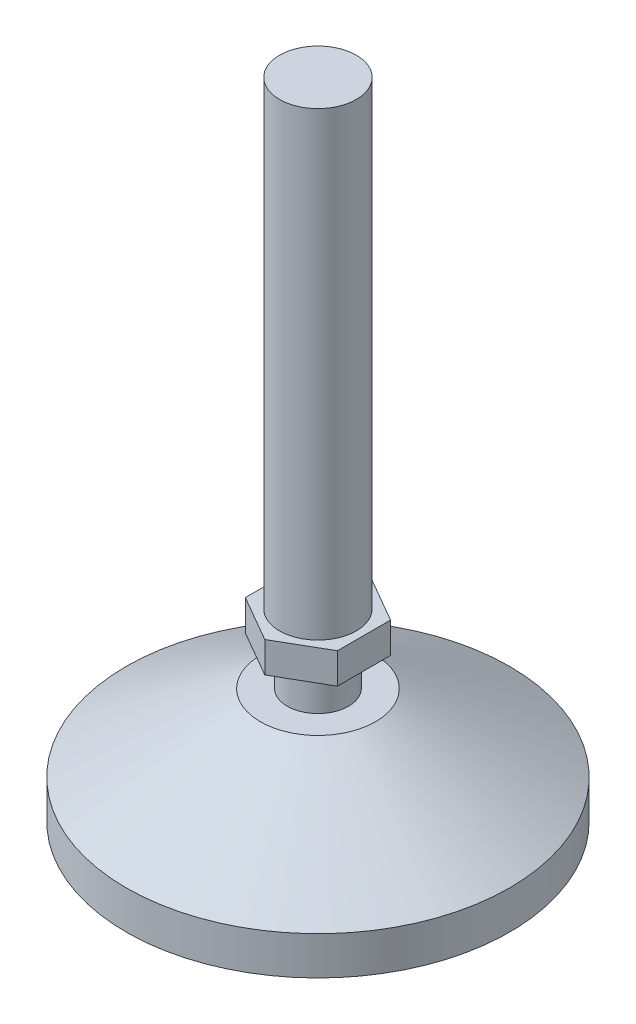
from build123d import *

# Parameters (mm, degrees)
SKETCH_2_R      = 8
EXTRUDE_1_DEPTH = 10
EXTRUDE_2_DEPTH = 8
SKETCH_4_R      = 10
EXTRUDE_3_DEPTH = 120


with BuildPart() as part:
    # 草图1 → 旋转1 (revolve)
    with BuildSketch(Plane.XY, mode=Mode.PRIVATE) as revolve_1_sk:
        Polygon((0, 30), (0, 0), (50, 0), (50, 10), (15, 30), align=None)
    revolve(revolve_1_sk.sketch.rotate(Axis((0, 30, 0), (0, -1, 0)), 180), axis=Axis((0, 30, 0), (0, -1, 0)))

    # 草图2 → 凸台-拉伸1 (add)
    with BuildSketch(Plane(origin=(0, 30, 0), x_dir=(1, 0, 0), z_dir=(0, 1, 0))):
        Circle(SKETCH_2_R)
    extrude(amount=EXTRUDE_1_DEPTH)

    # 草图3 → 凸台-拉伸2 (add)
    with BuildSketch(Plane(origin=(0, 40, 0), x_dir=(1, 0, 0), z_dir=(0, 1, 0))):
        Polygon((0, 13.856406461), (-12, 6.92820323), (-12, -6.92820323), (0, -13.856406461), (12, -6.92820323), (12, 6.92820323), align=None)
    extrude(amount=EXTRUDE_2_DEPTH)

    # 草图4 → 凸台-拉伸3 (add)
    with BuildSketch(Plane(origin=(0, 48, 0), x_dir=(1, 0, 0), z_dir=(0, 1, 0))):
        with Locations(Location((0, 0, 0), (0, 0, 270))):
            Circle(SKETCH_4_R)
    extrude(amount=EXTRUDE_3_DEPTH)


solid = part.part
